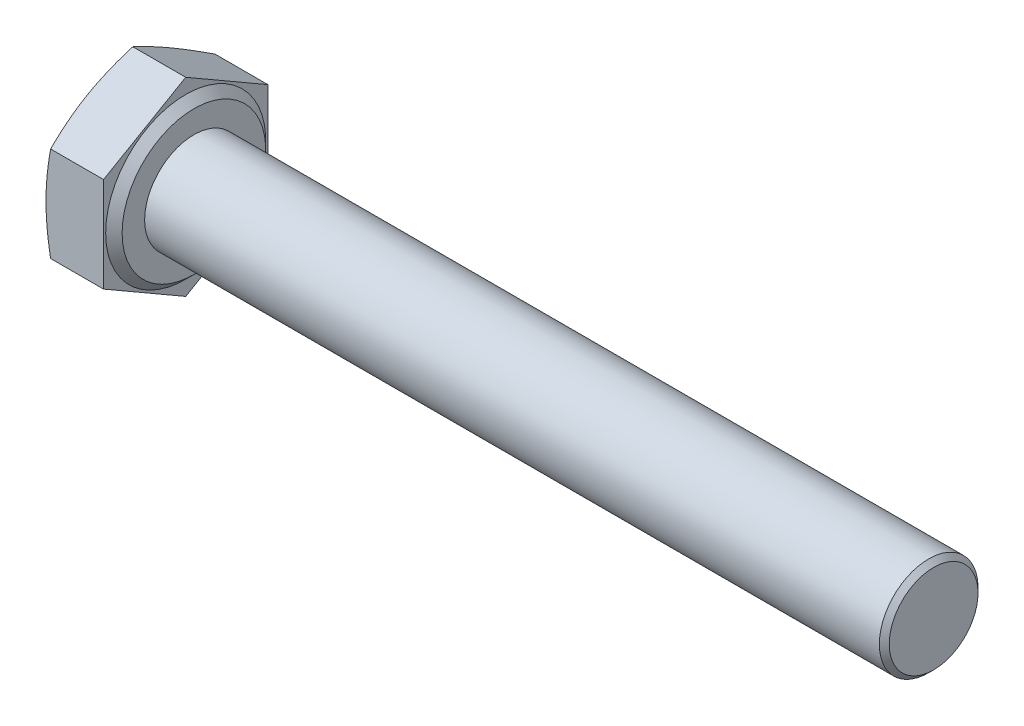
SolidWorks part; units mm, degrees
ref_plane "Front" through (0, 0, 0) normal (0, 0, 1) x (1, 0, 0)
ref_plane "Top" through (0, 0, 0) normal (0, 1, 0) x (1, 0, 0)
ref_plane "Right" through (0, 0, 0) normal (1, 0, 0) x (0, 0, -1)
other "Configuration Table"
sketch "Sketch2" plane through (0, 0, 0) normal (1, 0, 0) x (0, 0, -1)
  line L1 (0, -5.7735) -> (5, -2.8868)
  line L2 (5, -2.8868) -> (5, 2.8868)
  line L3 (5, 2.8868) -> (0, 5.7735)
  line L4 (0, 5.7735) -> (-5, 2.8868)
  line L5 (-5, 2.8868) -> (-5, -2.8868)
  line L6 (-5, -2.8868) -> (0, -5.7735)
  circle A0 centre (0, 0) radius 5 construction
extrude "BaseHead" add sketch "Sketch2" along normal blind 4
sketch "Sketch3" plane through (0, 0, 0) normal (0, 0, 1) x (1, 0, 0)
  line L0 (4, 5.7735) -> (4, 4.37)
  line L2 (4, 4.37) -> (3.5, 4.87)
  line L3 (3.5, 4.87) -> (3.5, 5.7735)
  line L5 (3.5, 5.7735) -> (4, 5.7735)
  line L6 (-0.9571, 0) -> (7.6478, 0) construction
  line L7 (4, 5.7735) -> (0, 5.7735) construction
  dimension "D1" = 45
  dimension "c" = 0.5
  dimension "dw" = 8.74
revolve "BearingFace" cut sketch "Sketch3" angle 360 about L6
sketch "Sketch4" plane through (0, 0, 0) normal (0, 0, 1) x (1, 0, 0)
  line L0 (-0.4935, 0) -> (3.5626, 0) construction
  line L2 (0, 5.7735) -> (0.2815, 5.7735)
  line L4 (0.2815, 5.7735) -> (0, 5)
  line L6 (0, 5) -> (0, 5.7735)
  line L7 (3.5, 5.7735) -> (0, 5.7735) construction
revolve "HeadChamfer" cut sketch "Sketch4" angle 360 about L0
sketch "Sketch5" plane through (4, 0, 0) normal (1, 0, 0) x (0, 0, -1)
  circle A0 centre (0, 0) radius 3
extrude "BaseBody" add sketch "Sketch5" along normal blind 45
cosmetic thread "ThreadCosmetic1" [suppressed] parameters "D2"=4.917
chamfer "Chamfer1" distance 0.3 angle 45 1 edges at (49, 0, -3)
fillet "HeadFillet" [suppressed] radius 0.25
sketch "Sketch6" plane through (0, 0, 0) normal (0, 0, 1) x (1, 0, 0)
  line L0 (4, 3.5415) -> (4.5415, 3.5415)
  line L1 (4.5415, 3.5415) -> (4.5415, 3)
  line L2 (4.5415, 3) -> (4.2708, 2.531)
  line L3 (4.2708, 2.531) -> (4, 3)
  line L4 (4, 3) -> (4, 3.5415)
  line L5 (4, -4.37) -> (4, 4.37) construction
  line L6 (48.7, 3) -> (4, 3) construction
revolve "Cut-Revolve10" [suppressed] cut sketch "Sketch6" angle 360
pattern_linear "LPattern10" [suppressed] count 69
equation "\"D2@Sketch4\" = \"s@Sketch2\""
equation "\"D1@Chamfer1\" = 0.05 * \"d@Sketch5\""
equation "\"D1@Sketch6\" =  ( \"d@Sketch5\" - \"D2@ThreadCosmetic1\" )  / 2"
equation "\"pitch@LPattern10\" = 1.2 * \"D1@Sketch6\""
equation "\"D1@LPattern10\" = (  \"l@BaseBody\"-\"D1@Chamfer1\" )  / \"pitch@LPattern10\""
